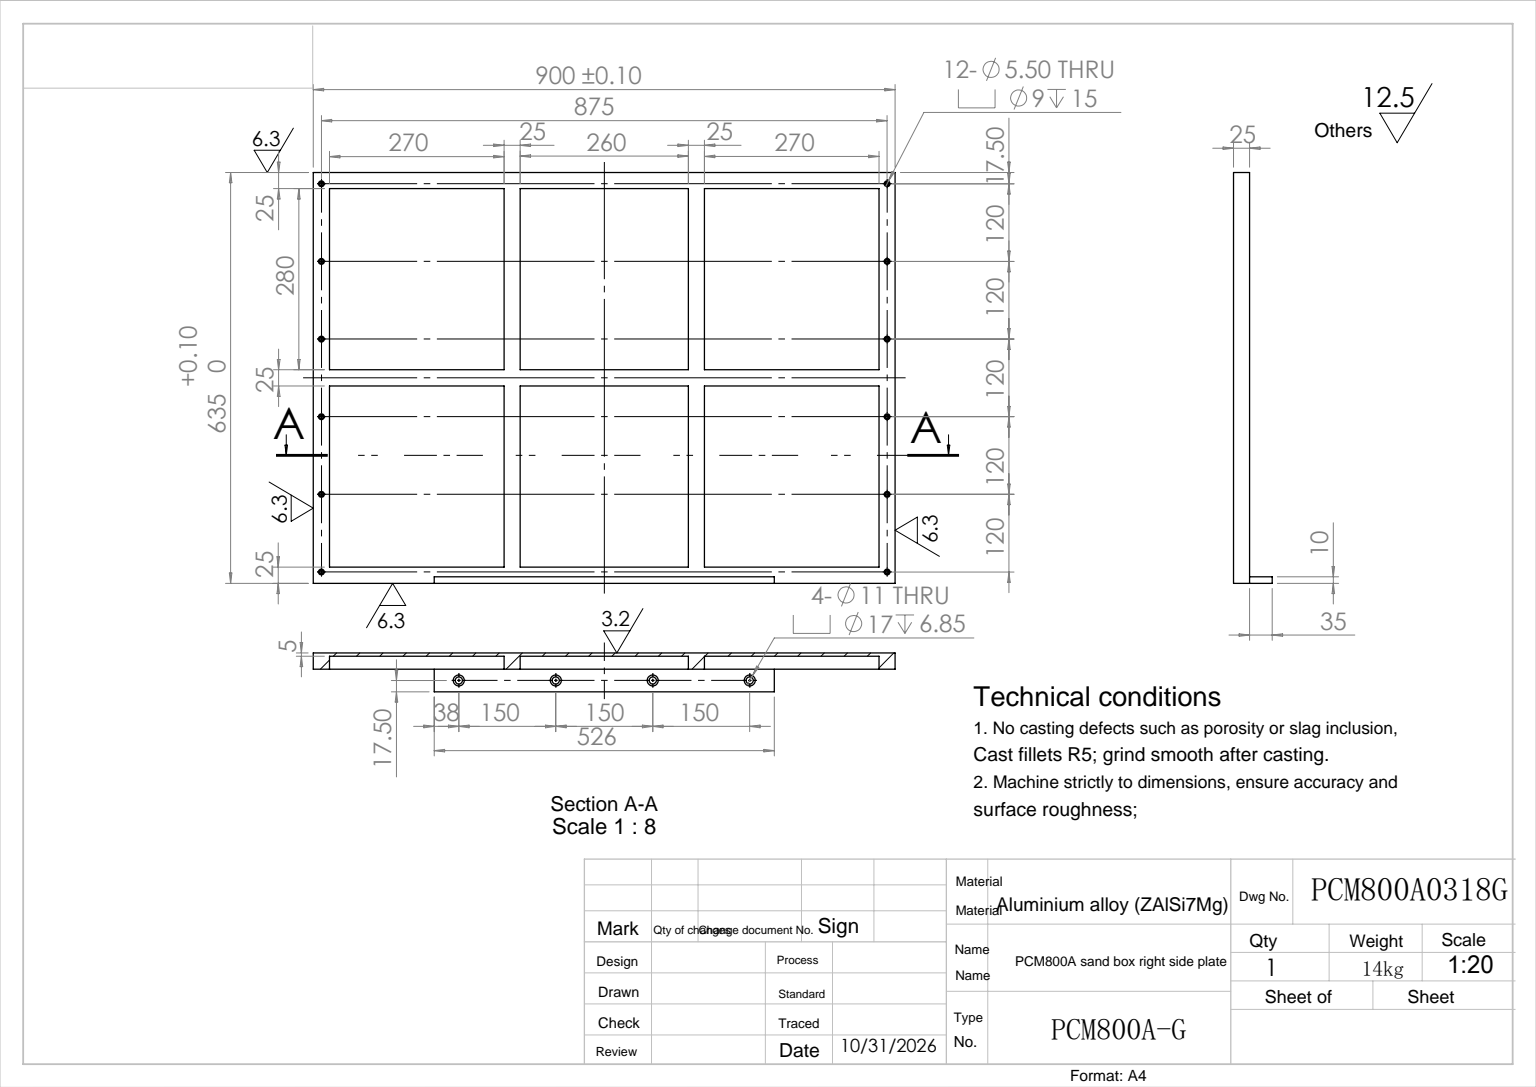
from build123d import *

# Parameters (mm, degrees)
SKETCH_1_W                = 900
SKETCH_1_H                = 635
EXTRUDE_1_DEPTH           = 5
SKETCH_2_W                = 25
SKETCH_2_H                = 635
EXTRUDE_2_DEPTH           = 20
SKETCH_4_W                = 850
SKETCH_4_H                = 25
EXTRUDE_3_DEPTH           = 20
SKETCH_5_W                = 25
SKETCH_5_H                = 585
EXTRUDE_4_DEPTH           = 20
SKETCH_6_W                = 850
SKETCH_6_H                = 25
EXTRUDE_5_DEPTH           = 20
SKETCH_7_W                = 526
SKETCH_7_H                = 10
EXTRUDE_6_DEPTH           = 35
HOLE_WIZARD_1_D           = 11
HOLE_WIZARD_1_CBORE_D     = 17
HOLE_WIZARD_1_CBORE_DEPTH = 6.85
HOLE_WIZARD_2_D           = 5.5
HOLE_WIZARD_2_CBORE_D     = 9
HOLE_WIZARD_2_CBORE_DEPTH = 15


with BuildPart() as part:
    # 草图1 → 拉伸1 (new body)
    with BuildSketch(Plane(origin=(0, 0, 0), x_dir=(0, 0, -1), z_dir=(1, 0, 0))):
        with Locations((450, 317.5)):
            Rectangle(SKETCH_1_W, SKETCH_1_H)
    extrude(amount=EXTRUDE_1_DEPTH)

    # 草图2 → 拉伸2 (add)
    with BuildSketch(Plane(origin=(5, 0, 0), x_dir=(0, 0, -1), z_dir=(1, 0, 0))):
        with Locations((12.5, 317.5)):
            Rectangle(SKETCH_2_W, SKETCH_2_H)
        with Locations((887.5, 317.5)):
            Rectangle(SKETCH_2_W, SKETCH_2_H)
    extrude(amount=EXTRUDE_2_DEPTH)

    # 草图4 → 拉伸3 (add)
    with BuildSketch(Plane(origin=(5, 0, 0), x_dir=(0, 0, -1), z_dir=(1, 0, 0))):
        with Locations((450, 622.5)):
            Rectangle(SKETCH_4_W, SKETCH_4_H)
        with Locations((450, 12.5)):
            Rectangle(SKETCH_4_W, SKETCH_4_H)
    extrude(amount=EXTRUDE_3_DEPTH)

    # 草图5 → 拉伸4 (add)
    with BuildSketch(Plane(origin=(5, 0, 0), x_dir=(0, 0, -1), z_dir=(1, 0, 0))):
        with Locations((307.5, 317.5)):
            Rectangle(SKETCH_5_W, SKETCH_5_H)
        with Locations((592.5, 317.5)):
            Rectangle(SKETCH_5_W, SKETCH_5_H)
    extrude(amount=EXTRUDE_4_DEPTH)

    # 草图6 → 拉伸5 (add)
    with BuildSketch(Plane(origin=(5, 0, 0), x_dir=(0, 0, -1), z_dir=(1, 0, 0))):
        with Locations((450, 317.5)):
            Rectangle(SKETCH_6_W, SKETCH_6_H)
    extrude(amount=EXTRUDE_5_DEPTH)

    # 草图7 → 拉伸6 (add)
    with BuildSketch(Plane(origin=(25, 0, 0), x_dir=(0, 0, -1), z_dir=(1, 0, 0))):
        with Locations((450, 5)):
            Rectangle(SKETCH_7_W, SKETCH_7_H)
    extrude(amount=EXTRUDE_6_DEPTH)

    # 孔1 (through all)
    with Locations(Plane(origin=(42.5, 10, -675), x_dir=(0, 0, 1), z_dir=(0, 1, 0))):
        with Locations((0, 0), (150, 0), (300, 0), (450, 0)):
            CounterBoreHole(HOLE_WIZARD_1_D / 2, HOLE_WIZARD_1_CBORE_D / 2, HOLE_WIZARD_1_CBORE_DEPTH)

    # 孔2 (through all)
    with Locations(Plane(origin=(25, 617.5, -12.5), x_dir=(0, 0, 1), z_dir=(1, 0, 0))):
        with Locations((0, 0), (0, 120), (0, 240), (0, 360), (0, 480), (0, 600)):
            hole_wizard_2 = CounterBoreHole(HOLE_WIZARD_2_D / 2, HOLE_WIZARD_2_CBORE_D / 2, HOLE_WIZARD_2_CBORE_DEPTH)

    # 镜向1: 孔2 across plane
    add(hole_wizard_2.mirror(Plane.XY.offset(-450)), mode=Mode.SUBTRACT)


solid = part.part
